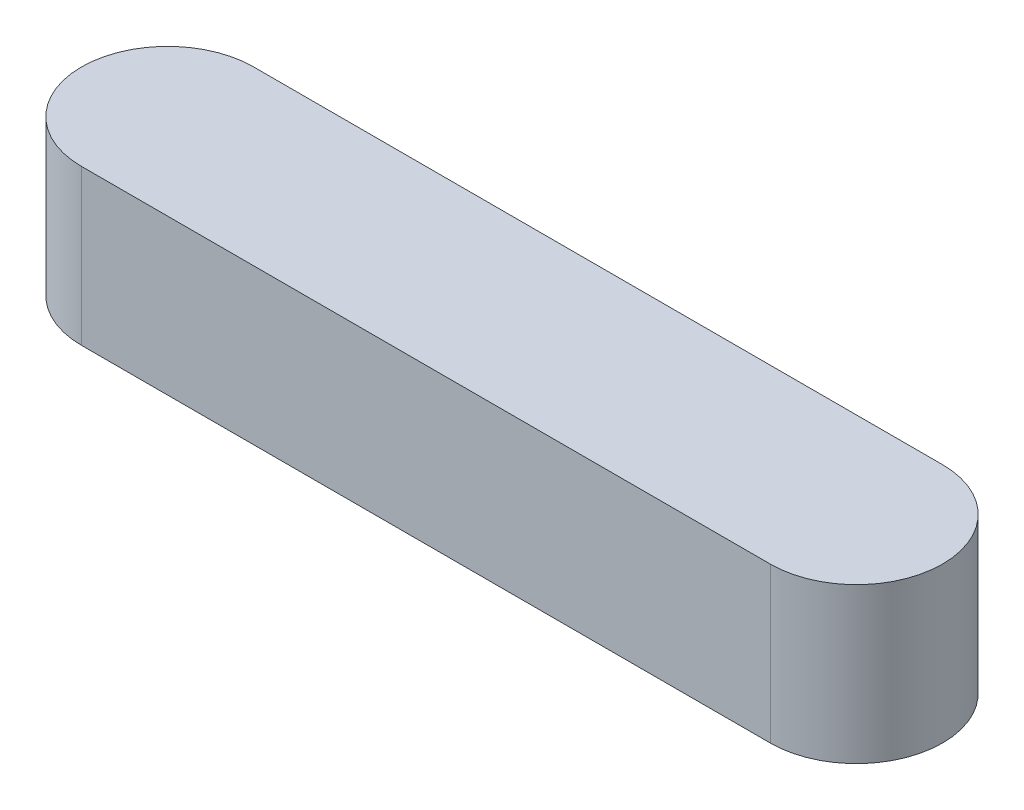
from build123d import *

# Parameters (mm, degrees)
BOSS_EXTRUDE1_DEPTH = 4.5


with BuildPart() as part:
    # Sketch1 → Boss-Extrude1 (new body)
    with BuildSketch(Plane(origin=(0, 0, 0), x_dir=(1, 0, 0), z_dir=(0, 1, 0))):
        with BuildLine():
            Line((-10, 2.5), (10, 2.5))
            ThreePointArc((10, 2.5), (12.5, 0), (10, -2.5))
            Line((10, -2.5), (-10, -2.5))
            ThreePointArc((-10, -2.5), (-12.5, 0), (-10, 2.5))
        make_face()
    extrude(amount=BOSS_EXTRUDE1_DEPTH)


solid = part.part
